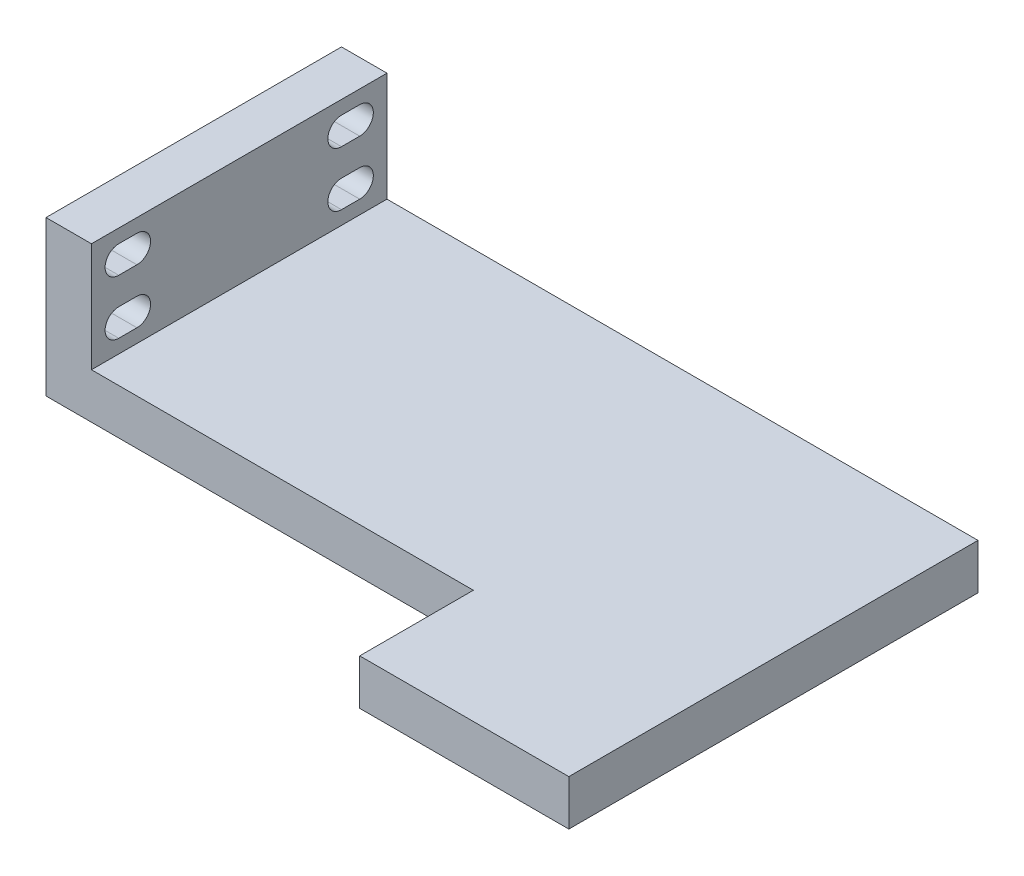
from build123d import *

# Parameters (mm, degrees)
EXTRUDE_1_DEPTH     = 32.5
CUT_EXTRUDE_1_REACH = 140.247
SKETCH_3_W          = 46
SKETCH_3_H          = 25
EXTRUDE_2_DEPTH     = 10


with BuildPart() as part:
    # 草图1 → 凸台-拉伸1 (new, symmetric)
    with BuildSketch(Plane.XY):
        Polygon((0, 0), (0, 34), (10, 34), (10, 10), (140, 10), (140, 0), align=None)
    extrude(amount=EXTRUDE_1_DEPTH, both=True)

    # 草图2 → 切除-拉伸1 (cut, up to next)
    with BuildSketch(Plane(origin=(10, 0, 0), x_dir=(0, 0, -1), z_dir=(1, 0, 0)), mode=Mode.PRIVATE) as cut_extrude_1_sk1:
        with BuildLine():
            Line((-26.5, 31), (-22.5, 31))
            ThreePointArc((-22.5, 31), (-19.5, 28), (-22.5, 25))
            Line((-22.5, 25), (-26.5, 25))
            ThreePointArc((-26.5, 25), (-29.5, 28), (-26.5, 31))
        make_face()
    cut_extrude_1_tool1 = extrude(cut_extrude_1_sk1.sketch, amount=-CUT_EXTRUDE_1_REACH, mode=Mode.PRIVATE) & part.part
    # 草图2 → 切除-拉伸1 (cut, up to next)
    with BuildSketch(Plane(origin=(10, 0, 0), x_dir=(0, 0, -1), z_dir=(1, 0, 0)), mode=Mode.PRIVATE) as cut_extrude_1_sk2:
        with BuildLine():
            Line((22.5, 31), (26.5, 31))
            ThreePointArc((26.5, 31), (29.5, 28), (26.5, 25))
            Line((26.5, 25), (22.5, 25))
            ThreePointArc((22.5, 25), (19.5, 28), (22.5, 31))
        make_face()
    cut_extrude_1_tool2 = extrude(cut_extrude_1_sk2.sketch, amount=-CUT_EXTRUDE_1_REACH, mode=Mode.PRIVATE) & part.part
    # 草图2 → 切除-拉伸1 (cut, up to next)
    with BuildSketch(Plane(origin=(10, 0, 0), x_dir=(0, 0, -1), z_dir=(1, 0, 0)), mode=Mode.PRIVATE) as cut_extrude_1_sk3:
        with BuildLine():
            Line((-26.5, 13), (-22.5, 13))
            ThreePointArc((-22.5, 13), (-19.5, 16), (-22.5, 19))
            Line((-22.5, 19), (-26.5, 19))
            ThreePointArc((-26.5, 19), (-29.5, 16), (-26.5, 13))
        make_face()
    cut_extrude_1_tool3 = extrude(cut_extrude_1_sk3.sketch, amount=-CUT_EXTRUDE_1_REACH, mode=Mode.PRIVATE) & part.part
    # 草图2 → 切除-拉伸1 (cut, up to next)
    with BuildSketch(Plane(origin=(10, 0, 0), x_dir=(0, 0, -1), z_dir=(1, 0, 0)), mode=Mode.PRIVATE) as cut_extrude_1_sk4:
        with BuildLine():
            Line((22.5, 13), (26.5, 13))
            ThreePointArc((26.5, 13), (29.5, 16), (26.5, 19))
            Line((26.5, 19), (22.5, 19))
            ThreePointArc((22.5, 19), (19.5, 16), (22.5, 13))
        make_face()
    cut_extrude_1_tool4 = extrude(cut_extrude_1_sk4.sketch, amount=-CUT_EXTRUDE_1_REACH, mode=Mode.PRIVATE) & part.part
    add(cut_extrude_1_tool1.solids().sort_by_distance((10, 28, 24.5))[0], mode=Mode.SUBTRACT)
    add(cut_extrude_1_tool2.solids().sort_by_distance((10, 28, -24.5))[0], mode=Mode.SUBTRACT)
    add(cut_extrude_1_tool3.solids().sort_by_distance((10, 16, 24.5))[0], mode=Mode.SUBTRACT)
    add(cut_extrude_1_tool4.solids().sort_by_distance((10, 16, -24.5))[0], mode=Mode.SUBTRACT)

    # 草图3 → 凸台-拉伸2 (add)
    with BuildSketch(Plane(origin=(0, 10, 0), x_dir=(1, 0, 0), z_dir=(0, 1, 0))):
        with Locations((117, -45)):
            Rectangle(SKETCH_3_W, SKETCH_3_H)
    extrude(amount=-EXTRUDE_2_DEPTH)


solid = part.part
